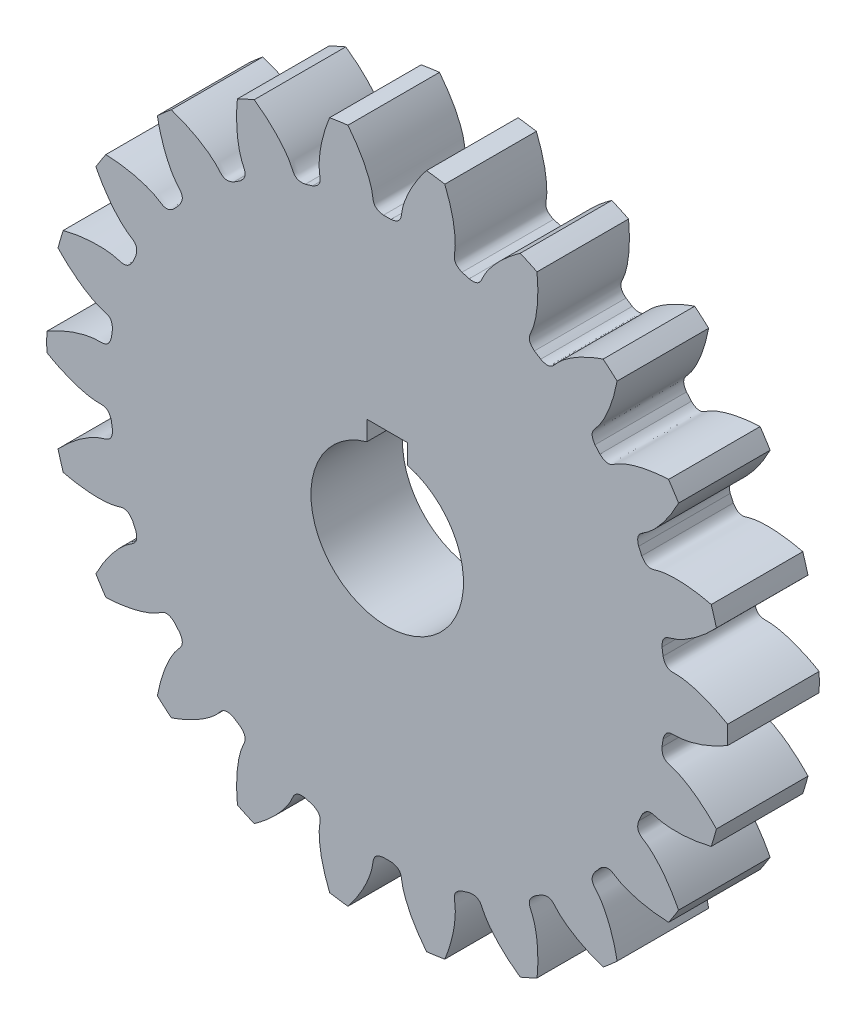
from build123d import *

# Parameters (mm, degrees)
SKETCH_1_R               = 66.940975
EXTRUDE_1_DEPTH          = 18
CUT_EXTRUDE_1_DEPTH      = 97.364870507
PATTERN_CIRCULAR_1_COUNT = 22
CUT_EXTRUDE_2_DEPTH      = 97.054702544


with BuildPart() as part:
    # 草图1 → 凸台-拉伸1 (new body)
    with BuildSketch(Plane.XY):
        Circle(SKETCH_1_R)
    extrude(amount=EXTRUDE_1_DEPTH)

    # 草图2 → 切除-拉伸1 (cut, through all)
    with BuildSketch(Plane.XY):
        with BuildLine():
            ThreePointArc((0.732201589, 54.679122808), (0, 54.684025), (-0.732201589, 54.679122808))
            add(Edge.make_bspline(
                [(-0.732201589, 54.679122808), (-2.825940324, 54.938964611), (-2.713580783, 56.139910127), (-2.933484179, 57.338429447), (-2.967490837, 57.505568946), (-3.009831884, 57.694178914), (-3.061336761, 57.903995913), (-3.122881524, 58.134716205), (-3.195316383, 58.386014559), (-3.279487764, 58.657538576), (-3.376230526, 58.948910768), (-3.486369459, 59.259728254), (-3.610717942, 59.589563202), (-3.750077478, 59.937963078), (-3.905236971, 60.304450964), (-4.076972088, 60.688525882), (-4.266044614, 61.089663137), (-4.473201811, 61.507314676), (-4.69917579, 61.940909459), (-4.944682897, 62.389853853), (-5.210423098, 62.853532036), (-5.497079382, 63.331306417), (-5.805317174, 63.822518073), (-6.135783753, 64.326487198), (-6.489107688, 64.842513571), (-6.865898282, 65.369877033), (-7.266745024, 65.907837983), (-7.692217065, 66.45563788), (-8.142862689, 67.012499773), (-8.619208814, 67.577628824), (-9.121760495, 68.150212865), (-9.651000444, 68.729422949), (-10.207388565, 69.314413927), (-10.791361498, 69.904325029), (-11.403332184, 70.498280459), (-12.043689441, 71.095390001), (-12.712797552, 71.694749639), (-13.410995876, 72.295442181), (-14.138598457, 72.896537899), (-14.895893712, 73.497095174), (-15.683143881, 74.096161164), (-16.785312332, 74.900580839), (-17.639368003, 75.485066142), (-18.222466845, 75.867592028)],
                knots=[0, 0, 0, 0, 0.118994009, 0.124264639, 0.130346134, 0.137238496, 0.144941724, 0.153455818, 0.162780778, 0.172916604, 0.183863296, 0.195620854, 0.208189278, 0.221568568, 0.235758725, 0.250759747, 0.266571636, 0.28319439, 0.300628011, 0.318872497, 0.33792785, 0.357794069, 0.378471154, 0.399959105, 0.422257922, 0.445367605, 0.469288154, 0.49401957, 0.519561851, 0.545914998, 0.573079012, 0.601053892, 0.629839637, 0.659436249, 0.689843727, 0.721062071, 0.75309128, 0.785931356, 0.819582299, 0.854044107, 0.889316781, 0.925400321, 1, 1, 1, 1], degree=3))
            ThreePointArc((-18.222466845, 75.867592028), (0, 78.025315238), (18.222466845, 75.867592028))
            add(Edge.make_bspline(
                [(0.732201589, 54.679122808), (2.825940324, 54.938964611), (2.713580783, 56.139910127), (2.933484179, 57.338429447), (2.967490837, 57.505568946), (3.009831884, 57.694178914), (3.061336761, 57.903995913), (3.122881524, 58.134716205), (3.195316383, 58.386014559), (3.279487764, 58.657538576), (3.376230526, 58.948910768), (3.486369459, 59.259728254), (3.610717942, 59.589563202), (3.750077478, 59.937963078), (3.905236971, 60.304450964), (4.076972088, 60.688525882), (4.266044614, 61.089663137), (4.473201811, 61.507314676), (4.69917579, 61.940909459), (4.944682897, 62.389853853), (5.210423098, 62.853532036), (5.497079382, 63.331306417), (5.805317174, 63.822518073), (6.135783753, 64.326487198), (6.489107688, 64.842513571), (6.865898282, 65.369877033), (7.266745024, 65.907837983), (7.692217065, 66.45563788), (8.142862689, 67.012499773), (8.619208814, 67.577628824), (9.121760495, 68.150212865), (9.651000444, 68.729422949), (10.207388565, 69.314413927), (10.791361498, 69.904325029), (11.403332184, 70.498280459), (12.043689441, 71.095390001), (12.712797552, 71.694749639), (13.410995876, 72.295442181), (14.138598457, 72.896537899), (14.895893712, 73.497095174), (15.683143881, 74.096161164), (16.785312332, 74.900580839), (17.639368003, 75.485066142), (18.222466845, 75.867592028)],
                knots=[0, 0, 0, 0, 0.118994009, 0.124264639, 0.130346134, 0.137238496, 0.144941724, 0.153455818, 0.162780778, 0.172916604, 0.183863296, 0.195620854, 0.208189278, 0.221568568, 0.235758725, 0.250759747, 0.266571636, 0.28319439, 0.300628011, 0.318872497, 0.33792785, 0.357794069, 0.378471154, 0.399959105, 0.422257922, 0.445367605, 0.469288154, 0.49401957, 0.519561851, 0.545914998, 0.573079012, 0.601053892, 0.629839637, 0.659436249, 0.689843727, 0.721062071, 0.75309128, 0.785931356, 0.819582299, 0.854044107, 0.889316781, 0.925400321, 1, 1, 1, 1], degree=3))
        make_face()
    cut_extrude_1 = extrude(amount=CUT_EXTRUDE_1_DEPTH, mode=Mode.SUBTRACT)

    # 阵列(圆周)1: 切除-拉伸1 ×22 about axis
    pattern_circular_1_axis = Axis((0, 0, 18), (0, 0, -1))
    for i in range(1, PATTERN_CIRCULAR_1_COUNT):
        add(cut_extrude_1.rotate(pattern_circular_1_axis, i * 360 / PATTERN_CIRCULAR_1_COUNT), mode=Mode.SUBTRACT)

    # 草图4 → 切除-拉伸2 (cut, through all)
    with BuildSketch(Plane.XY.offset(18)):
        with BuildLine():
            Line((-4, 18.3), (4, 18.3))
            Line((4, 18.3), (4, 14.456832295))
            ThreePointArc((4, 14.456832295), (0, -15), (-4, 14.456832295))
            Line((-4, 14.456832295), (-4, 18.3))
        make_face()
    extrude(amount=-CUT_EXTRUDE_2_DEPTH, mode=Mode.SUBTRACT)


solid = part.part
